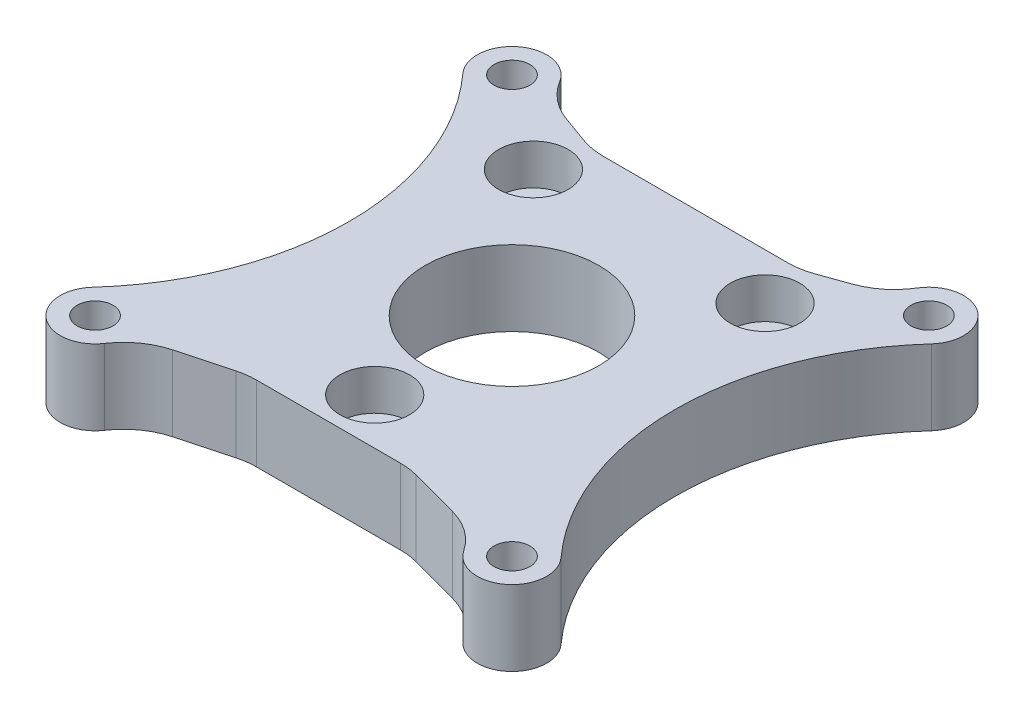
SolidWorks part; units mm, degrees
material "尼龙 101"
ref_plane "前视基准面" through (0, 0, 0) normal (0, 0, 1) x (1, 0, 0)
ref_plane "上视基准面" through (0, 0, 0) normal (0, 1, 0) x (1, 0, 0)
ref_plane "右视基准面" through (0, 0, 0) normal (1, 0, 0) x (0, 0, -1)
other "Configuration Table"
sketch "草图1" plane through (0, 0, 0) normal (0, 1, 0) x (1, 0, 0)
  line L0 (0, 0) -> (0, 25.5968) construction
  line L1 (-18, 18) -> (18, 18) construction
  line L2 (-18, 18) -> (-18, -18) construction
  line L3 (-18, -18) -> (18, -18) construction
  line L4 (18, 18) -> (18, -18) construction
  line L5 (-18, 18) -> (18, -18) construction
  line L6 (-18, -18) -> (18, 18) construction
  line L7 (0, 0) -> (74.5, 0) construction
  line L8 (74.5, 0) -> (74.5, 36.9227) construction
  line L9 (167, -18) -> (131, 18) construction
  line L10 (167, 18) -> (131, -18) construction
  line L11 (131, 18) -> (131, -18) construction
  line L12 (167, -18) -> (131, -18) construction
  line L13 (167, 18) -> (167, -18) construction
  line L14 (167, 18) -> (131, 18) construction
  line L16 (-10, 11.85) -> (10, 11.85) construction
  line L17 (10, 11.85) -> (0, -11.85) construction
  line L18 (0, -11.85) -> (-10, 11.85) construction
  line L19 (-15, 18) -> (-9, 15.85)
  line L20 (-9, 15.85) -> (9, 15.85)
  line L21 (7, -15.85) -> (-7, -15.85)
  line L22 (-7, -15.85) -> (-15, -18)
  line L23 (7, -15.85) -> (15, -18)
  line L24 (15, 18) -> (9, 15.85)
  line L25 (134, 18) -> (140, 15.85) construction
  line L26 (158, 15.85) -> (140, 15.85) construction
  line L27 (164, 18) -> (158, 15.85) construction
  line L28 (142, -15.85) -> (134, -18) construction
  line L29 (142, -15.85) -> (156, -15.85) construction
  line L30 (156, -15.85) -> (164, -18) construction
  circle A0 centre (18, 18) radius 1.55
  circle A1 centre (18, -18) radius 1.55
  circle A2 centre (-18, -18) radius 1.55
  circle A3 centre (-18, 18) radius 1.55
  circle A4 centre (10, 11.85) radius 1.55 construction
  circle A5 centre (0, -11.85) radius 1.55 construction
  circle A6 centre (-10, 11.85) radius 1.55 construction
  circle A8 centre (37.875, 0) radius 22 construction
  circle A9 centre (111.125, 0) radius 22 construction
  circle A10 centre (159, 11.85) radius 1.55 construction
  circle A11 centre (149, -11.85) radius 1.55 construction
  circle A12 centre (139, 11.85) radius 1.55 construction
  circle A13 centre (167, 18) radius 1.55 construction
  circle A14 centre (167, -18) radius 1.55 construction
  circle A15 centre (131, -18) radius 1.55 construction
  circle A16 centre (131, 18) radius 1.55 construction
  arc A17 (-15, 18) -> (-20.2236, 15.9862) centre (-18, 18) ccw
  arc A18 (20.2236, 15.9862) -> (15, 18) centre (18, 18) ccw
  arc A19 (15, -18) -> (20.2236, -15.9862) centre (18, -18) ccw
  arc A20 (-20.2236, -15.9862) -> (-15, -18) centre (-18, -18) ccw
  arc A21 (20.2236, 15.9862) -> (20.2236, -15.9862) centre (37.875, 0) ccw
  arc A22 (-20.2236, 15.9862) -> (-20.2236, -15.9862) centre (-37.875, 0) cw
  circle A23 centre (0, 0) radius 7.5 construction
  circle A24 centre (-10, 11.85) radius 3 construction
  circle A25 centre (0, -11.85) radius 3 construction
  arc A26 (128.7764, 15.9862) -> (134, 18) centre (131, 18) cw construction
  arc A27 (128.7764, 15.9862) -> (128.7764, -15.9862) centre (111.125, 0) cw construction
  arc A28 (134, -18) -> (128.7764, -15.9862) centre (131, -18) cw construction
  circle A29 centre (149, 0) radius 7.5 construction
  arc A30 (169.2236, -15.9862) -> (164, -18) centre (167, -18) cw construction
  arc A31 (169.2236, 15.9862) -> (169.2236, -15.9862) centre (186.875, 0) ccw construction
  arc A32 (164, 18) -> (169.2236, 15.9862) centre (167, 18) cw construction
  point P0 (0, 0)
  point P40 (149, 0)
  point P54 (0, -15.85)
  point P57 (0, 15.85)
  dimension "D2" = 3.1
  dimension "D3" = 10
  dimension "D4" = 11.85
  dimension "D5" = 23.7
  dimension "D6" = 44
  dimension "D9" = 6
  dimension "D14" = 15
  dimension "D15" = 6
  dimension "D16" = 6
  dimension "D1" = 36
  dimension "D7" = 56.5
  dimension "D8" = 36.625
  dimension "D10" = 4
  dimension "D11" = 6
  dimension "D12" = 4
  dimension "D13" = 8
extrude "凸台-拉伸1" add sketch "草图1" along normal blind 6.5
fillet "圆角1" radius 6 8 edges at (-15, 3.25, -18) (-15, 3.25, 18) (-7, 3.25, 15.85) (7, 3.25, 15.85) (15, 3.25, 18) (-9, 3.25, -15.85) (9, 3.25, -15.85) (15, 3.25, -18)
sketch "草图9" plane through (0, 6.5, 0) normal (0, 1, 0) x (1, 0, 0)
  line L0 (0, 0) -> (0, 19.7579) construction
  line L1 (0, 0) -> (18.6177, 0) construction
  circle A0 centre (0, 0) radius 7.5
  circle A1 centre (10, 11.85) radius 1.55
  circle A2 centre (0, -11.85) radius 1.55
  circle A3 centre (-10, 11.85) radius 1.55
  dimension "D1" = 15
  dimension "D2" = 3.1
  dimension "D3" = 10
  dimension "D4" = 11.85
  dimension "D5" = 23.7
extrude "切除-拉伸11" cut sketch "草图9" against normal through all
sketch "草图10" plane through (0, 6.5, 0) normal (0, 1, 0) x (1, 0, 0)
  circle A0 centre (-10, 11.85) radius 3
  circle A1 centre (10, 11.85) radius 3
  circle A2 centre (0, -11.85) radius 3
  dimension "D1" = 6
extrude "切除-拉伸12" cut sketch "草图10" against normal blind 3.5
